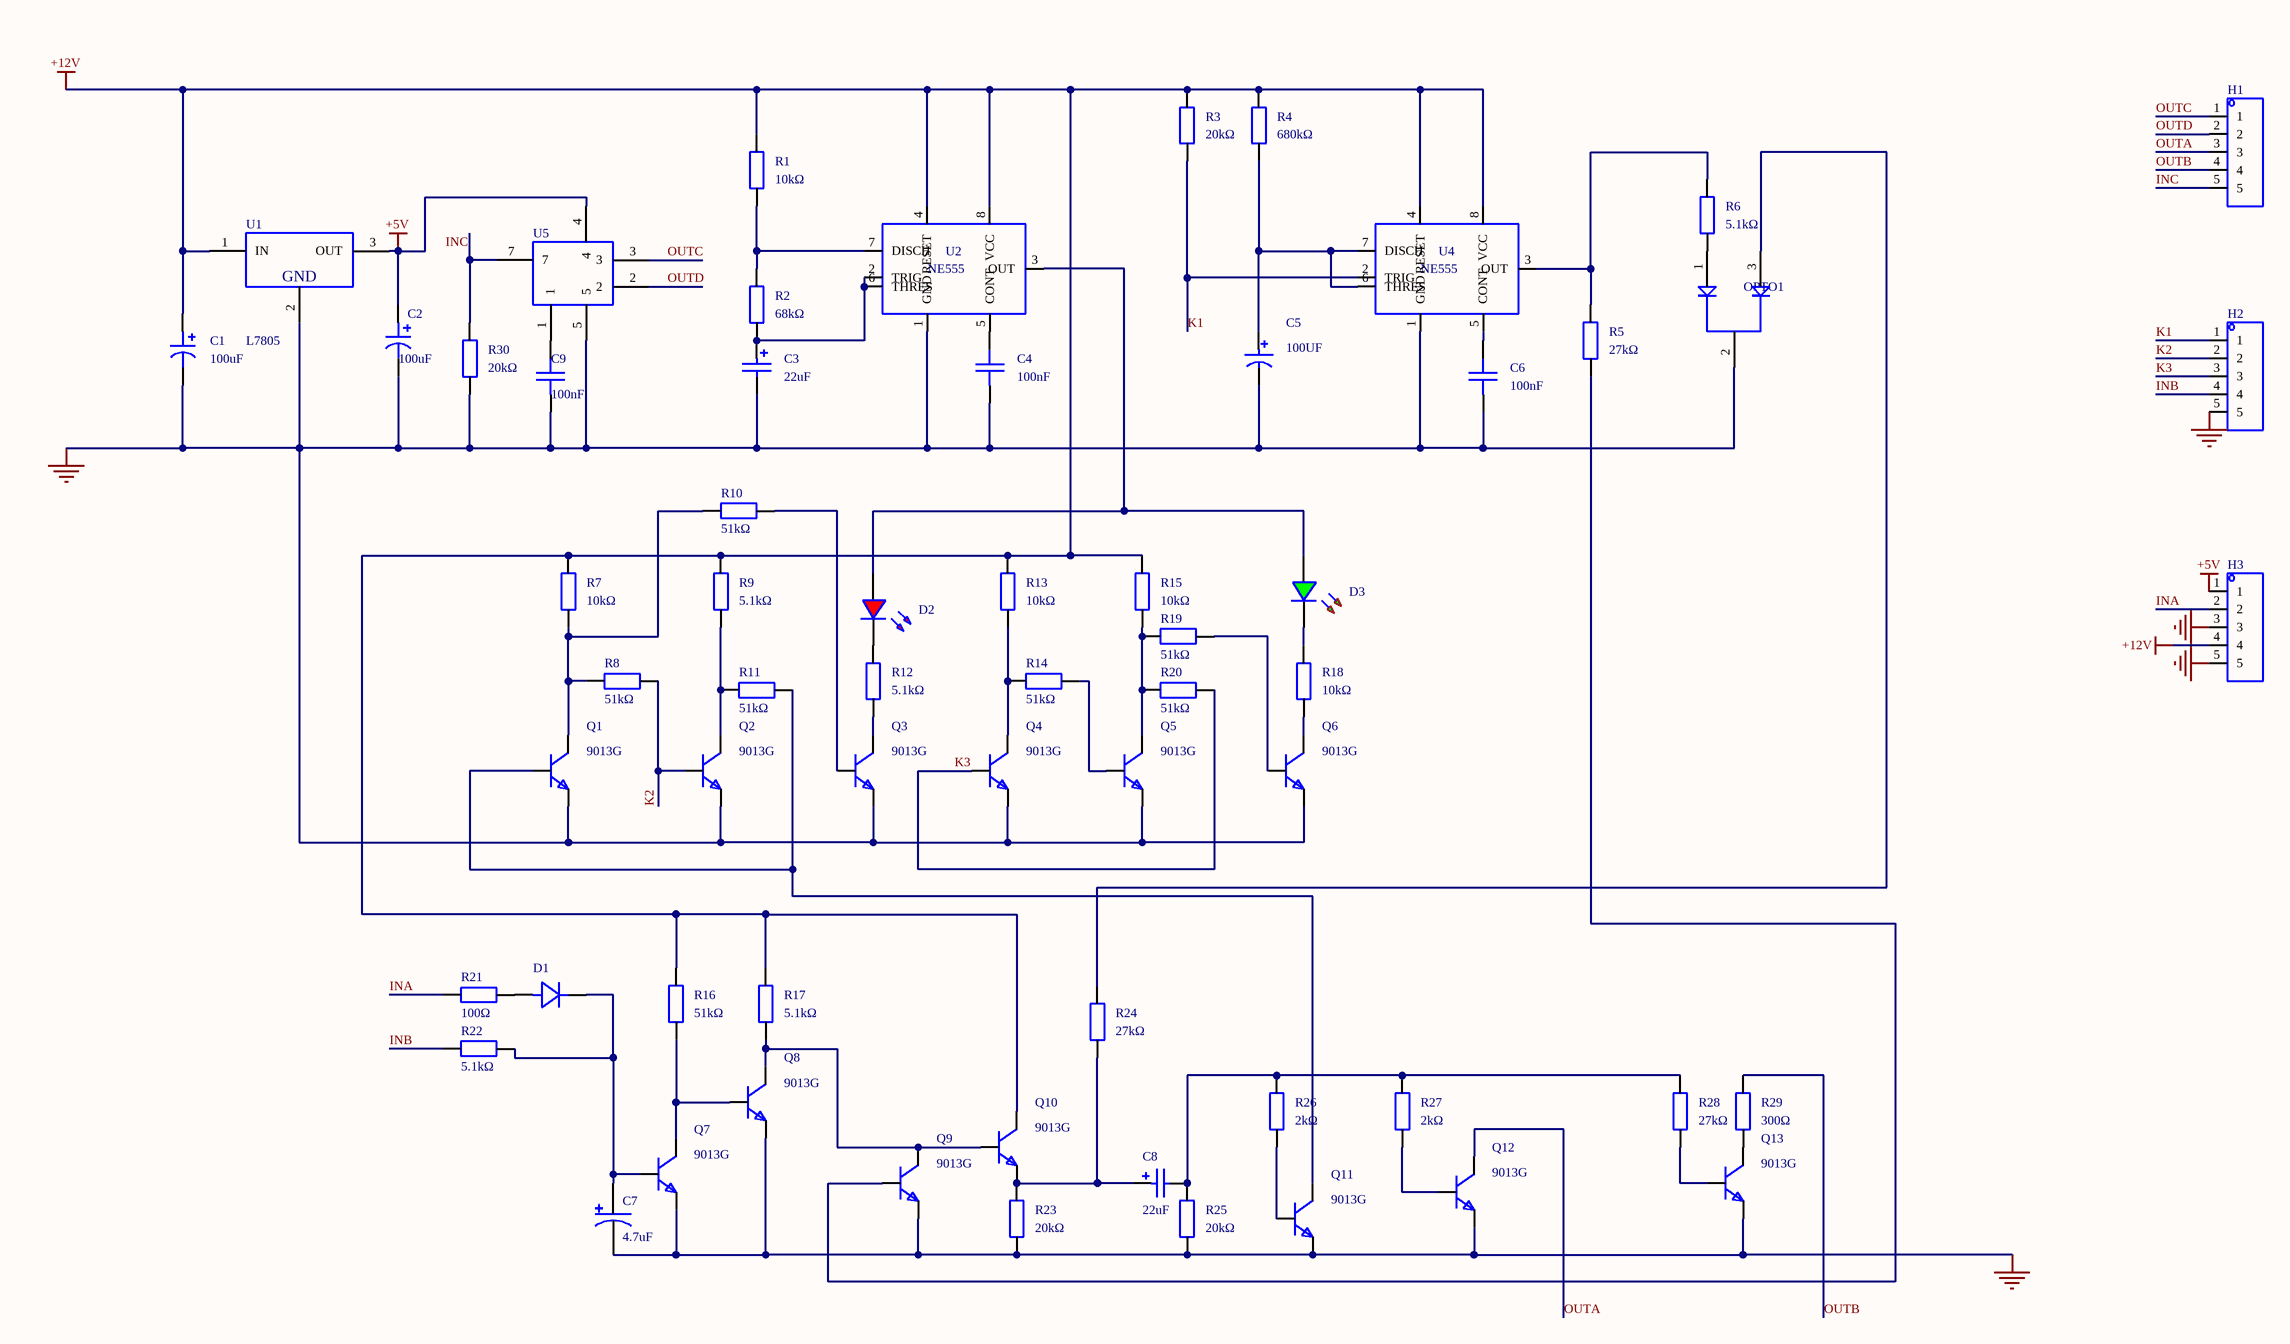
[diagram p0: MISC89097-3.schdoc]
# Altium project MISC89097-2.PrjPcb
1 sheet, 63 parts. Net scope: global (net labels, ports and power ports of the same name join across sheets).
Board file: MISC89097.pcbdoc

## Sheet MISC89097-3.schdoc
size 178 x 98 mm; Version: V1.0; @Project Name: MISC89097; @Page Count: 1; @Update Date: 2025-01-04; @Create Date: 2025-01-04; @Schematic Name: MISC89097; @Page No: 1; @Board Name: MISC89097; @Create Time: 19:46:02; @Update Time: 19:13:31

### Parts
C1  100uF  [CAP-TH_BD8.0-P3.50-D0.6-FD_1]
C2  100uF  [CAP-TH_BD8.0-P3.50-D0.6-FD_1]
C3  22uF  [CAP-TH_BD5.0-P2.5-D0.5-FD]
C4  100nF  [CAP-TH_L5.0-W2.5-P5.00-D1.0]
C5  100UF  [CAP-TH_BD5.0-P2.00-D0.8-FD]
C6  100nF  [CAP-TH_L5.0-W2.5-P5.00-D1.0]
C7  4.7uF  [CAP-TH_BD6.3-P2.50-D1.0-FD]
C8  22uF  [CAP-TH_BD5.0-P2.5-D0.5-FD]
C9  100nF  [CAP-TH_L5.0-W2.5-P5.00-D1.0]
D1  (no value)  [DO_1N4007]
D2  (no value)  [LED-TH_5mm]
D3  (no value)  [LED-TH_5mm]
H1  (no value)  [HDR-TH_5P-P2.54-V-M]
H2  (no value)  [HDR-TH_5P-P2.54-V-M]
H3  (no value)  [HDR-TH_5P-P2.54-V-M]
OPTO1  38K infrared receiver, side-mounted  [OPTO-TH_3P-BD5.9-P2.54]  (value not drawn)
Q1  9013G  [TO-92-3_L4.9-W3.7-P1.27-L]
Q2  9013G  [TO-92-3_L4.9-W3.7-P1.27-L]
Q3  9013G  [TO-92-3_L4.9-W3.7-P1.27-L]
Q4  9013G  [TO-92-3_L4.9-W3.7-P1.27-L]
Q5  9013G  [TO-92-3_L4.9-W3.7-P1.27-L]
Q6  9013G  [TO-92-3_L4.9-W3.7-P1.27-L]
Q7  9013G  [TO-92-3_L4.9-W3.7-P1.27-L]
Q8  9013G  [TO-92-3_L4.9-W3.7-P1.27-L]
Q9  9013G  [TO-92-3_L4.9-W3.7-P1.27-L]
Q10  9013G  [TO-92-3_L4.9-W3.7-P1.27-L]
Q11  9013G  [TO-92-3_L4.9-W3.7-P1.27-L]
Q12  9013G  [TO-92-3_L4.9-W3.7-P1.27-L]
Q13  9013G  [TO-92-3_L4.9-W3.7-P1.27-L]
R1  10kΩ  [Res_1/4W]
R2  68kΩ  [Res_1/4W]
R3  20kΩ  [Res_1/4W]
R4  680kΩ  [Res_1/4W]
R5  27kΩ  [Res_1/4W]
R6  5.1kΩ  [Res_1/4W]
R7  10kΩ  [Res_1/4W]
R8  51kΩ  [Res_1/4W]
R9  5.1kΩ  [Res_1/4W]
R10  51kΩ  [Res_1/4W]
R11  51kΩ  [Res_1/4W]
R12  5.1kΩ  [Res_1/4W]
R13  10kΩ  [Res_1/4W]
R14  51kΩ  [Res_1/4W]
R15  10kΩ  [Res_1/4W]
R16  51kΩ  [Res_1/4W]
R17  5.1kΩ  [Res_1/4W]
R18  10kΩ  [Res_1/4W]
R19  51kΩ  [Res_1/4W]
R20  51kΩ  [Res_1/4W]
R21  100Ω  [Res_1/4W]
R22  5.1kΩ  [Res_1/4W]
R23  20kΩ  [Res_1/4W]
R24  27kΩ  [Res_1/4W]
R25  20kΩ  [Res_1/4W]
R26  2kΩ  [Res_1/4W]
R27  2kΩ  [Res_1/4W]
R28  27kΩ  [Res_1/4W]
R29  300Ω  [Res_1/4W]
R30  20kΩ  [Res_1/4W]
U1  L7805  [TO-220AB-3_L10.4-W4.6-P2.54-L]
U2  NE555  [PDIP-8_L9.6-W6.4-P2.54-LS7.9-BL-1]
U4  NE555  [PDIP-8_L9.6-W6.4-P2.54-LS7.9-BL-1]
U5  (no value)  [DIP-8_L9.9-W6.4-P2.54-LS7.6-BL]

### Nets
+5V: C2.1 H3.1 U1.3(OUT) U5.4
+12V: C1.1 H3.4 Q10.3(C) R1.2 R3.2 R4.2 R7.2 R9.2 R13.2 R15.2 R16.1 R17.1 U1.1(IN) U2.4(RESET) U2.8(VCC) U4.4(RESET) U4.8(VCC)
GND: C1.2 C2.2 C3.2 C4.2 C5.2 C6.2 C7.2 C9.2 H2.5 H3.3 H3.5 OPTO1.2 Q1.1(E) Q2.1(E) Q3.1(E) Q4.1(E) Q5.1(E) Q6.1(E) Q7.1(E) Q8.1(E) Q9.1(E) Q11.1(E) Q12.1(E) Q13.1(E) R23.2 R25.2 R30.1 U1.2(GND) U2.1(GND) U4.1(GND) U5.5
INA: H3.2 R21.2
INB: H2.4 R22.2
INC: H1.5 R30.2 U5.7
K1: H2.1 R3.1 U4.2(TRIG)
K2: H2.2 Q2.2(B) R8.1
K3: H2.3 Q4.2(B) R20.1
OUTA: H1.3 Q12.3(C)
OUTB: H1.4 R29.1
OUTC: H1.1 U5.3
OUTD: H1.2 U5.2
NetC3_1: C3.1 R2.1 U2.2(TRIG) U2.6(THRES)
NetC4_1: C4.1 U2.5(CONT)
NetC5_1: C5.1 R4.1 U4.6(THRES) U4.7(DISCH)
NetC6_1: C6.1 U4.5(CONT)
NetC7_1: C7.1 D1.1(K) Q7.2(B) R22.1
NetC8_1: C8.1 Q10.1(E) R23.1 R24.2
NetC8_2: C8.2 R25.1 R26.1 R27.1 R28.1
NetC9_1: C9.1 U5.1
NetD1_2: D1.2(A) R21.1
NetD2_1: D2.1(C) D3.1(C) U2.3(OUT)
NetD2_2: D2.2(A) R12.2
NetD3_2: D3.2(A) R18.2
NetOPTO1_1: OPTO1.1 R6.1
NetOPTO1_3: OPTO1.3 R24.1
NetQ1_2: Q1.2(B) Q11.3(C) R11.1
NetQ1_3: Q1.3(C) R7.1 R8.2 R10.2
NetQ2_3: Q2.3(C) R9.1 R11.2
NetQ3_2: Q3.2(B) R10.1
NetQ3_3: Q3.3(C) R12.1
NetQ4_3: Q4.3(C) R13.1 R14.2
NetQ5_2: Q5.2(B) R14.1
NetQ5_3: Q5.3(C) R15.1 R19.2 R20.2
NetQ6_2: Q6.2(B) R19.1
NetQ6_3: Q6.3(C) R18.1
NetQ7_3: Q7.3(C) Q8.2(B) R16.2
NetQ8_3: Q8.3(C) Q9.3(C) Q10.2(B) R17.2
NetQ9_2: Q9.2(B) R5.1
NetQ11_2: Q11.2(B) R26.2
NetQ12_2: Q12.2(B) R27.2
NetQ13_2: Q13.2(B) R28.2
NetQ13_3: Q13.3(C) R29.2
NetR1_1: R1.1 R2.2 U2.7(DISCH)
NetR5_2: R5.2 R6.2 U4.3(OUT)

### Notes on the sheet
- 2025-01-04
- Schematic
- Sheet
- Material code
- P1
- Checked
- Drawn
- Revision
- Size
- page
- Total
- A4
- 1

### Library data of the parts
C1 C2 = 100uF: Symbol: 100UF_C9900016884; AddInBom: yes; ModelId: 5fc21599cab34df2ad7753b19b2f5286; ModelTransform: 315.365,314.914,0,0,0,0,0,0,-196.85; Device: 100uF; LCSC Part Name: 100uF; SupplierPart: C9900016884; ManufacturerPart: 100uF; Supplier Footprint: CAP-TH_BD8.0-P3.50-D1.0-FD; JLCPCB Part Class: Extended library; Supplier: LCSC; ConvertToPcb: yes; FootprintName: CAP-TH_BD8.0-P3.50-D0.6-FD_1; ModelName: CAP-TH_BD8.0-P3.50-D0.6-FD_1
C3 C8 = TAP226K016SCS: Capacitance:22uF;Accuracy:±10%;Rated voltage:16V;ESR:2Ω@100kHz;; Manufacturer: Kyocera AVX; AddInBom: yes; ModelId: 5998369278cc462c87d4182ea76811bf; ModelName: CAP-TH_BD5.0-H7.5-P2.5; ModelTransform: 196.70055,196.77528,0,0,0,0,0,0,-137.795; Tolerance: ±10%; Rated Voltage: 16V; Symbol: TAP226K016SCS; Device: TAP226K016SCS; LCSC Part Name: 22uF ±10% 16V; SupplierPart: C62893; ManufacturerPart: TAP226K016SCS; Supplier Footprint: 插件,P=2.5mm; JLCPCB Part Class: Extended library; Datasheet: https://atta.szlcsc.com/upload/public/pdf/source/20191107/C444779_CCD9EA7F36AC07ADEC9ACFBB03523055.pdf; Supplier: LCSC; ConvertToPcb: yes; FootprintName: CAP-TH_BD5.0-P2.5-D0.5-FD; Value: 22uF; Equivalent Series Resistance(ESR): 2Ω@100kHz; Operating Temperature: -55℃~+125℃
C4 C6 C9 = 100nF: Symbol: 100NF_C9900015256; AddInBom: yes; ModelId: 08e3d7481fc7486bb1b263873f51e1e1; ModelName: CAP-TH_BD5.0-W2.5-P5.08; ModelTransform: 224.652,98.425,0,0,0,0,-0.005,0,-137.795; Device: 100nF; LCSC Part Name: 100nF; SupplierPart: C9900015256; ManufacturerPart: 100nF; Supplier Footprint: CAP-TH_L5.0-W2.5-P5.00-D1.0; JLCPCB Part Class: Extended library; Supplier: LCSC; ConvertToPcb: yes; FootprintName: CAP-TH_L5.0-W2.5-P5.00-D1.0
C5 = 0.1uF 50V 5*11: Capacitance:100nF;Rated voltage:50V;Ripple current:1A@100kHz;ESR:-;; AddInBom: yes; ModelId: edeeed87cbc746108d01291548c38636; ModelName: CAP-TH_D5.0×H7.0×P2.0; ModelTransform: 197.091,196.7911,0,0,0,0,0,0,-137.795; Rated Voltage: 50V; φD: 5mm; L: 11mm; Lifetime @ Temp: 1000hrs@105℃; Value: 100UF; Symbol: 0.1uF 50V 5*11; Device: 0.1uF 50V 5*11; LCSC Part Name: 100nF 50V; ManufacturerPart: 0.1uF 50V 5*11; Supplier Footprint: 插件,5x11mm; JLCPCB Part Class: Extended library; Supplier: LCSC; ConvertToPcb: yes; FootprintName: CAP-TH_BD5.0-P2.00-D0.8-FD; Ripple Current: 1A@100kHz; Equivalent Series Resistance(ESR): -; Lead Spacing: 2mm
C7 = LKMC1202G4R7MF: Capacitance:4.7uF;Accuracy:±20%;Rated voltage:400V;Ripple current:140mA@100kHz;ESR:23.5Ω@100kHz;; Manufacturer: Ymin(永铭); AddInBom: yes; ModelId: 0a4db4bf24b443b3be4905be97ff10c5; ModelTransform: 248.4247,247.99777,0,0,0,0,0,0,-137.795; Tolerance: ±20%; Rated Voltage: 400V; φD: 6.3mm; L: 12mm; Lifetime @ Temp: 9000hrs@105℃; Symbol: LKMC1202G4R7MF; Device: LKMC1202G4R7MF; LCSC Part Name: 4.7uF ±20% 400V; SupplierPart: C443285; ManufacturerPart: LKMC1202G4R7MF; Supplier Footprint: 插件,D6.3xL12mm; JLCPCB Part Class: Extended library; Datasheet: https://atta.szlcsc.com/upload/public/pdf/source/20200220/C487520_443A40905984A455D375EE990FEAA9E8.pdf; Supplier: LCSC; ConvertToPcb: yes; FootprintName: CAP-TH_BD6.3-P2.50-D1.0-FD; ModelName: CAP-TH_BD6.3-P2.50-D1.0-FD; Value: 4.7uF; Ripple Current: 140mA@100kHz; Equivalent Series Resistance(ESR): 23.5Ω@100kHz; Lead Spacing: 2.5mm
D1 = D_1N4007A: AddInBom: yes; ModelId: 6de1e9b71a0d4751b4e9df530304c1a3; ModelName: DO-41_D2.4-L4.7-P8.70; ModelTransform: 373.9,94.4,232.29,0,0,0,0,0,-140; Symbol: D_1N4007; Device: D_1N4007A; Supplier Footprint: DO-41; ConvertToPcb: yes; FootprintName: DO_1N4007
D2 = LED_TH-R_5mm: ConvertToPcb: yes; ModelId: fe9cea1bdf7642cd8d9a5077ed0e2b58; ModelName: LED-TH_BD5.9-P2.54-RD_RED; ModelTransform: 222.16,238.98,581.81,180,0,0,-6,0,-220; Symbol: LED_TH-R; Device: LED_TH-R_5mm; AddInBom: yes; FootprintName: LED-TH_5mm; Supplier Footprint: 插件
D3 = LED_TH-G_5mm: ConvertToPcb: yes; ModelId: fe7796f666a04da4b4289311169b45200819f05c4eef4c71ace90d822a990e87; ModelName: LED-TH_BD5.8-P2.54-FD_GREEN-1; ModelTransform: 212.58,227.91,537.36,0,0,0,-7.87,0,-196.85; Device: LED_TH-G_5mm; AddInBom: yes; Supplier Footprint: 插件; SymbolName: LED_TH-G; FootprintName: LED-TH_5mm
H1-H3 = HDR-M_2.54_1x5P: Symbol: MTP125-1105S1; ConvertToPcb: yes; ModelId: 47d466e4a34f4fc5bc626cf773a24dd5; ModelName: HDR-TH_5P-P2.54-M-LI-1X5P; ModelTransform: 499.999,100,0,0,0,0,0,0,-118.11; Device: HDR-M_2.54_1x5P; AddInBom: yes; SupplierPart: C358687; Supplier Footprint: 插件; FootprintName: HDR-TH_5P-P2.54-V-M
OPTO1 = 红外38K接收管-侧放: AddInBom: yes; ModelId: d08885393af84744923b23fc53e5db16; ModelTransform: 227.156,232.267,0,180,0,0,-1.969,-2.703,-196.85; Symbol: 38K infrared receiver, side-mounted; Device: 38K infrared receiver, side-mounted; LCSC Part Name: 红外38K接收管-侧放; SupplierPart: C9900017189; ManufacturerPart: 红外38K接收管-侧放; Supplier Footprint: 0038; JLCPCB Part Class: Extended library; Supplier: LCSC; ConvertToPcb: yes; FootprintName: OPTO-TH_3P-BD5.9-P2.54; ModelName: OPTO-TH_3P-BD5.9-P2.54
Q1-Q13 = 9013G: Manufacturer: ST(先科); AddInBom: yes; ModelId: db569d051dcd4484acf2f9e50678fca3; ModelTransform: 180.7872,141.4455,0,0,0,0,0,22.677,-196.85; Symbol: 9013G; Device: 9013G; LCSC Part Name: 9013G; SupplierPart: C2859143; ManufacturerPart: 9013G; Supplier Footprint: TO-92; JLCPCB Part Class: Extended library; Datasheet: https://atta.szlcsc.com/upload/public/pdf/source/20220902/8AB04C64396E52FAEDF5BDA5E4896788.pdf; Supplier: LCSC; ConvertToPcb: yes; FootprintName: TO-92-3_L4.9-W3.7-P1.27-L; ModelName: TO-92-3_L4.9-W3.7-P1.27-L
R1-R30 = Res_AXIAL-1/4W: Symbol: Resistor; AddInBom: yes; ModelId: 463263665006444ab7a47bd11b0cf956; ModelName: RES-TH_BD2.4-L6.3-P10.30-D0.6; ModelTransform: 427.165,94.32816,0,0,0,0,0,0,-196.85; Device: Res_AXIAL-1/4W; Supplier Footprint: 轴向引线; ConvertToPcb: yes; FootprintName: Res_1/4W
  R1 R7 R13 R15 R18: Value: 10kΩ
  R2: Value: 68kΩ
  R3 R23 R25 R30: Value: 20kΩ
  R4: Value: 680kΩ
  R5 R24 R28: Value: 27kΩ
  R6 R9 R12 R17 R22: Value: 5.1kΩ
  R8 R10 R11 R14 R16 R19 R20: Value: 51kΩ
  R21: Value: 100Ω
  R26 R27: Value: 2kΩ
  R29: Value: 300Ω
U1 = L7805: Fixed output; positive polarity; max input voltage 35V; output voltage 5V; output current 1.2A; ripple rejection (PSRR) 62dB@(120Hz); Manufacturer: SY(顺烨）; AddInBom: yes; ModelId: d1d0dbd076494fbeaa52623fe55fdf16; ModelName: TO-220AB_3PIN-L10.5-W5.0-H20.0-P2.54; ModelTransform: 413.385,191.3382,0,0,0,0,-0.001,25.592,-393.701; Symbol: L7805; Device: L7805; LCSC Part Name: L7805; SupplierPart: C7426851; ManufacturerPart: L7805; Supplier Footprint: TO-220AB; Datasheet: https://atta.szlcsc.com/upload/public/pdf/source/20230613/EFD68926364DD51E58BF6EC5864FDDFA.pdf; Supplier: LCSC; ConvertToPcb: yes; FootprintName: TO-220AB-3_L10.4-W4.6-P2.54-L
U2 U4 = NE555PE4: Single-precision timer 8-PDIP 0 to 70; Manufacturer: TI(德州仪器); AddInBom: yes; ModelId: 1b8eaf096e7944deafe216467068c10e; ModelTransform: 377.952,318.897,0,0,0,0,0,0,-118.11; Manufacturer Part: NE555; Symbol: NE555PE4; Device: NE555PE4; LCSC Part Name: NE555PE4; SupplierPart: C2859604; Supplier Footprint: PDIP-8; JLCPCB Part Class: Extended library; Datasheet: ADDRESS_REDACTED; Supplier: LCSC; ConvertToPcb: yes; FootprintName: PDIP-8_L9.6-W6.4-P2.54-LS7.9-BL-1; ModelName: PDIP-8_L9.6-W6.4-P2.54-LS7.9-BL-1
U5 = 语音模块sop-8: Device: Voice module, sop-8; AddInBom: yes; ConvertToPcb: yes; SymbolName: Voice module, sop-8